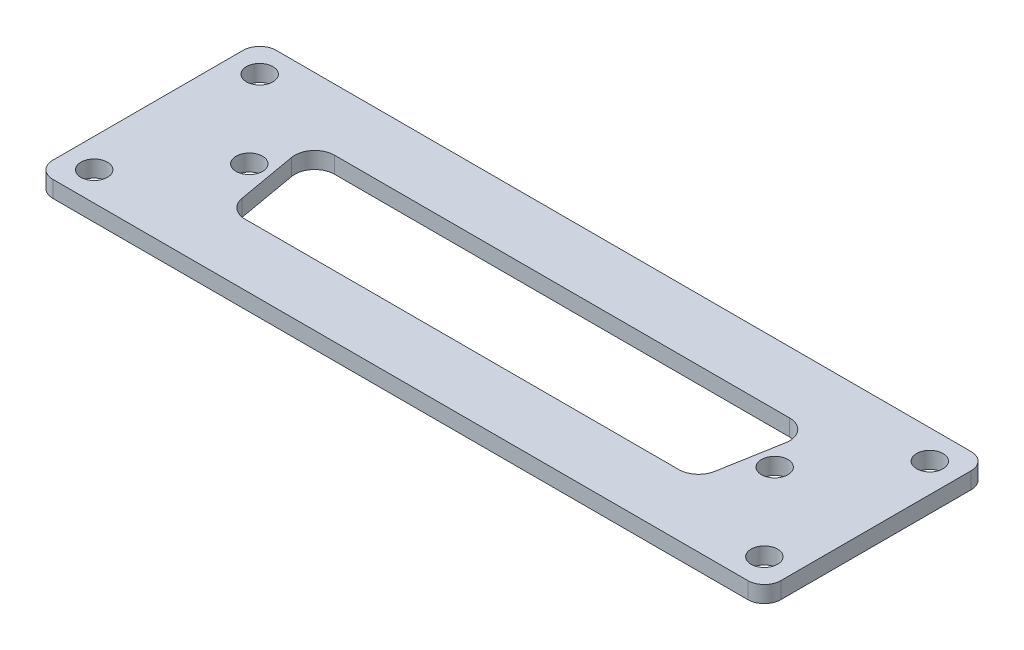
SolidWorks part; units mm, degrees
ref_plane "Front Plane" through (0, 0, 0) normal (0, 0, 1) x (1, 0, 0)
ref_plane "Top Plane" through (0, 0, 0) normal (0, 1, 0) x (1, 0, 0)
ref_plane "Right Plane" through (0, 0, 0) normal (1, 0, 0) x (0, 0, -1)
sketch "Sketch1" plane through (0, 0, 0) normal (0, 1, 0) x (1, 0, 0)
  line L1 (-44, -13.5) -> (44, -13.5)
  line L2 (-44, -13.5) -> (-44, 13.5)
  line L3 (-44, 13.5) -> (44, 13.5)
  line L4 (44, -13.5) -> (44, 13.5)
  line L5 (-44, -13.5) -> (44, 13.5) construction
  line L6 (-44, 13.5) -> (44, -13.5) construction
  point P0 (0, 0)
  dimension "D1" = 88
  dimension "D2" = 27
extrude "Boss-Extrude1" add sketch "Sketch1" along normal blind 2
sketch "Sketch2" plane through (0, 2, 0) normal (0, 1, 0) x (1, 0, 0)
  line L1 (-40.5, -10) -> (40.5, -10) construction
  line L2 (-40.5, -10) -> (-40.5, 10) construction
  line L3 (-40.5, 10) -> (40.5, 10) construction
  line L4 (40.5, -10) -> (40.5, 10) construction
  line L5 (-40.5, -10) -> (40.5, 10) construction
  line L6 (-40.5, 10) -> (40.5, -10) construction
  circle A0 centre (-40.5, 10) radius 1.6
  circle A1 centre (40.5, 10) radius 1.6
  circle A2 centre (40.5, -10) radius 1.6
  circle A3 centre (-40.5, -10) radius 1.6
  point P0 (0, 0)
  dimension "D3" = 3.2
  dimension "D4" = 3.2
  dimension "D5" = 3.2
  dimension "D6" = 3.2
  dimension "D1" = 20
  dimension "D2" = 81
extrude "Cut-Extrude1" cut sketch "Sketch2" against normal through all
fillet "Fillet1" radius 2 4 edges at (44, 1, -13.5) (44, 1, 13.5) (-44, 1, 13.5) (-44, 1, -13.5)
sketch "Sketch3" plane through (0, 2, 0) normal (0, 1, 0) x (1, 0, 0)
  line L0 (-29.5681, 3.2853) -> (-28.2809, -4.0147) construction
  line L1 (-26.2128, -5.75) -> (26.2128, -5.75) construction
  line L3 (-27.5, 5.75) -> (27.5, 5.75) construction
  line L5 (30.0027, 5.75) -> (30.0027, 9.1834) construction
  line L6 (-30.0027, 5.75) -> (-30.0027, 9.6921) construction
  line L7 (29.5681, 3.2853) -> (28.2809, -4.0147) construction
  line L8 (-29.8635, 3.2332) -> (-28.5764, -4.0668)
  line L9 (-26.2128, -6.05) -> (26.2128, -6.05)
  line L10 (29.8635, 3.2332) -> (28.5764, -4.0668)
  line L11 (-27.5, 6.05) -> (27.5, 6.05)
  arc A0 (28.2809, -4.0147) -> (26.2128, -5.75) centre (26.2128, -3.65) cw construction
  arc A1 (27.5, 5.75) -> (29.5681, 3.2853) centre (27.5, 3.65) cw construction
  arc A2 (-28.2809, -4.0147) -> (-26.2128, -5.75) centre (-26.2128, -3.65) ccw construction
  arc A3 (-29.5681, 3.2853) -> (-27.5, 5.75) centre (-27.5, 3.65) cw construction
  arc A4 (-28.5764, -4.0668) -> (-26.2128, -6.05) centre (-26.2128, -3.65) ccw
  arc A5 (28.5764, -4.0668) -> (26.2128, -6.05) centre (26.2128, -3.65) cw
  arc A6 (27.5, 6.05) -> (29.8635, 3.2332) centre (27.5, 3.65) cw
  arc A7 (-29.8635, 3.2332) -> (-27.5, 6.05) centre (-27.5, 3.65) cw
  point P0 (0, 0)
  dimension "D5" = 2.1
  dimension "D1" = 10
  dimension "D2" = 10
  dimension "D3" = 11.5
  dimension "D4" = 5.75
  dimension "D6" = 55
  dimension "D7" = 27.5
  dimension "D8" = 0.3
extrude "Cut-Extrude2" cut sketch "Sketch3" against normal through all
hole_wizard "M3 Tapped Hole1" positions "Sketch4" profile "Sketch5" tap size "M3" standard "GB" end condition through all
sketch "Sketch4" plane through (0, 2, 0) normal (0, 1, 0) x (1, 0, 0)
  point P2 (-31.75, 0)
  point P4 (31.75, 0)
  dimension "D1" = 63.5
  dimension "D2" = 31.75
sketch "Sketch5" plane through (-31.75, 2, 0) normal (1, 0, 0) x (0, 0, 1)
  line L0 (0, 0) -> (0, 2)
  line L1 (0, 2) -> (1.25, 2)
  line L2 (1.25, 2) -> (1.25, 0)
  line L5 (1.25, 0) -> (0, 0)
  line L11 (0, -6.35) -> (0, 107.95) construction
  dimension "通孔螺纹孔钻头直径" = 2.5
  dimension "通孔螺纹孔钻头深度" = 2
cosmetic thread "Hole Thread1" parameters "D2"=3
cosmetic thread "Hole Thread2" parameters "D2"=3
sketch "Sketch6" plane through (0, 2, 0) normal (0, 1, 0) x (1, 0, 0)
  circle A0 centre (-31.75, 0) radius 1.6
  circle A1 centre (31.75, 0) radius 1.6
  dimension "D1" = 3.2
  dimension "D2" = 3.2
extrude "Cut-Extrude3" cut sketch "Sketch6" against normal through all
